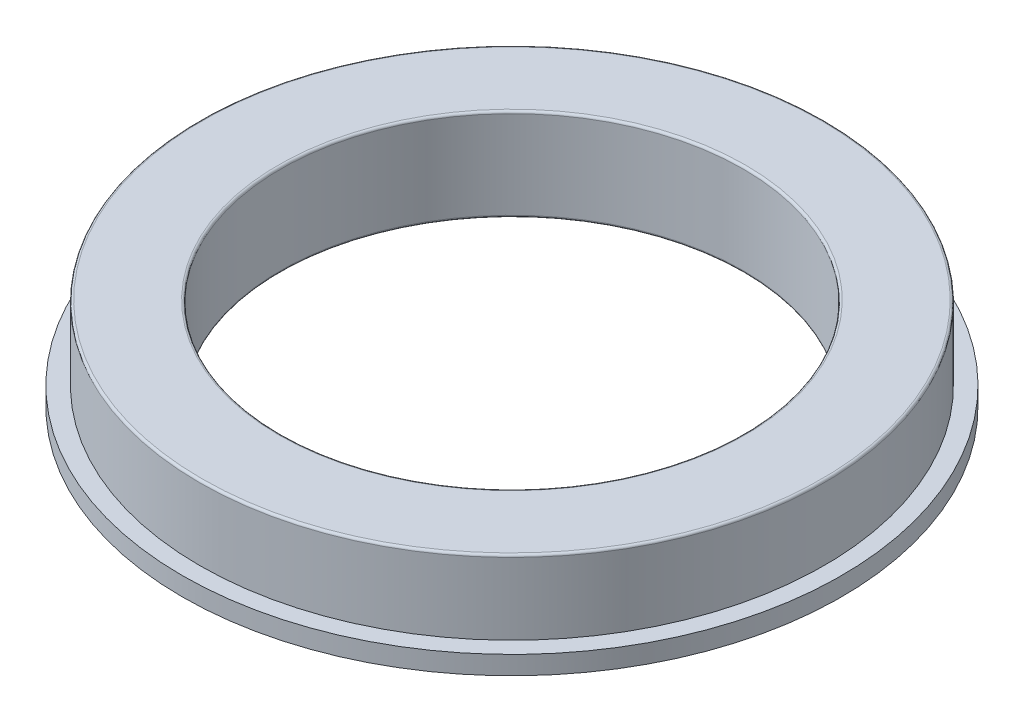
from build123d import *

# Parameters (mm, degrees)
SKETCH_1_R      = 14.25
SKETCH_1_R_2    = 10
EXTRUDE_1_DEPTH = 0.8
SKETCH_2_R      = 13.5
SKETCH_2_R_2    = 10
EXTRUDE_2_DEPTH = 3.2
FILLET_R0_1_1_R = 0.1


with BuildPart() as part:
    # 草图1 → 凸台-拉伸1 (new body)
    with BuildSketch(Plane(origin=(0, 0, 0), x_dir=(1, 0, 0), z_dir=(0, 1, 0))):
        with Locations(Location((0, 0, 0), (0, 0, 270))):
            Circle(SKETCH_1_R)
        with Locations(Location((0, 0, 0), (0, 0, 270))):
            Circle(SKETCH_1_R_2, mode=Mode.SUBTRACT)
    extrude(amount=EXTRUDE_1_DEPTH)

    # 草图2 → 凸台-拉伸2 (add)
    with BuildSketch(Plane(origin=(0, 0.8, 0), x_dir=(1, 0, 0), z_dir=(0, 1, 0))):
        with Locations(Location((0, 0, 0), (0, 0, 270))):
            Circle(SKETCH_2_R)
        with Locations(Location((0, 0, 0), (0, 0, 270))):
            Circle(SKETCH_2_R_2, mode=Mode.SUBTRACT)
    extrude(amount=EXTRUDE_2_DEPTH)

    # R0.1 圆角1
    fillet_r0_1_1_edges = [part.edges().sort_by_distance(p)[0] for p in [
        (0, 4, -13.5),
        (0, 4, -10),
        (0, 0, -10),
    ]]
    fillet(fillet_r0_1_1_edges, radius=FILLET_R0_1_1_R)


solid = part.part
